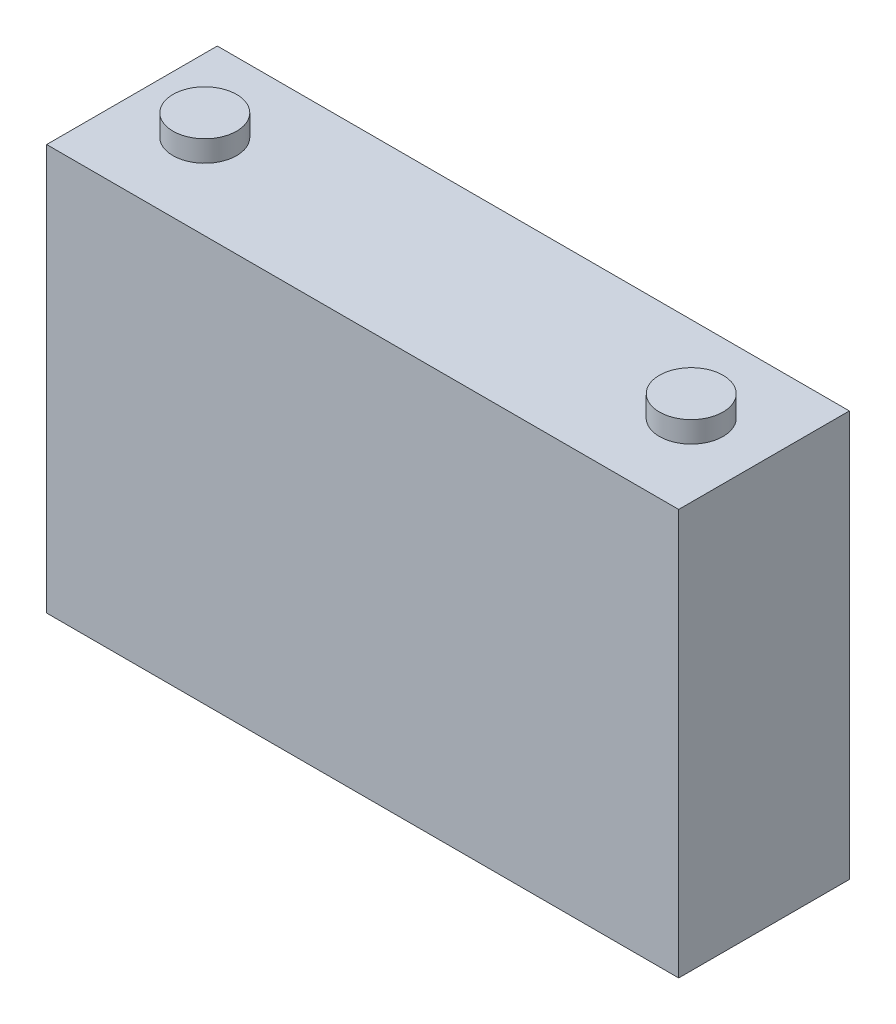
SolidWorks part; units mm, degrees
material "陶瓷"
ref_plane "前视基准面" through (0, 0, 0) normal (0, 0, 1) x (1, 0, 0)
ref_plane "上视基准面" through (0, 0, 0) normal (0, 1, 0) x (1, 0, 0)
ref_plane "右视基准面" through (0, 0, 0) normal (1, 0, 0) x (0, 0, -1)
sketch "草图1" plane through (0, 0, 0) normal (0, 1, 0) x (1, 0, 0)
  line L1 (-74.45, 20.1) -> (74.45, 20.1)
  line L2 (-74.45, 20.1) -> (-74.45, -20.1)
  line L3 (-74.45, -20.1) -> (74.45, -20.1)
  line L4 (74.45, 20.1) -> (74.45, -20.1)
  line L5 (-74.45, 20.1) -> (74.45, -20.1) construction
  line L6 (-74.45, -20.1) -> (74.45, 20.1) construction
  point P0 (0, 0)
  dimension "D1" = 40.2
  dimension "D2" = 148.9
extrude "凸台-拉伸1" add sketch "草图1" along normal blind 95.6
sketch "草图2" plane through (0, 95.6, 0) normal (0, 1, 0) x (1, 0, 0)
  line L0 (-57.3, 0) -> (57.3, 0) construction
  circle A0 centre (57.3, 0) radius 7.5
  circle A1 centre (-57.3, 0) radius 7.5
  dimension "D2" = 15
  dimension "D1" = 114.6
extrude "凸台-拉伸2" add sketch "草图2" along normal blind 5
